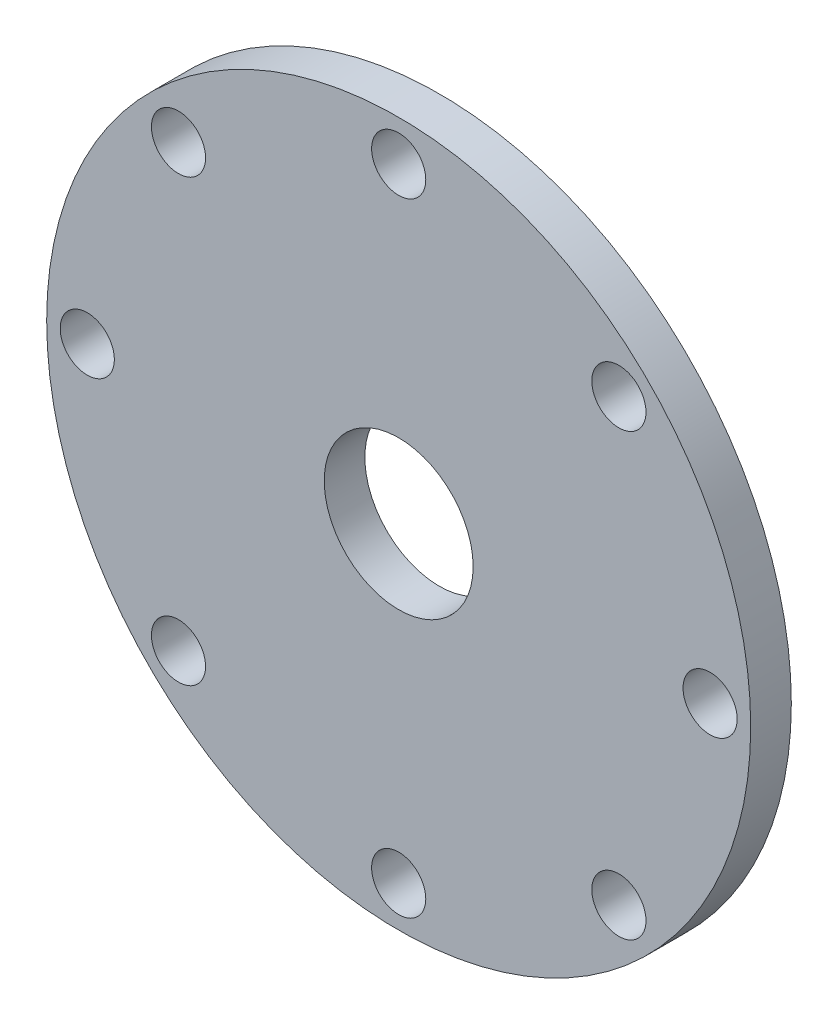
from build123d import *

# Parameters (mm, degrees)
SKETCH2_R           = 130
SKETCH2_R_2         = 27.5
BOSS_EXTRUDE1_DEPTH = 15
SKETCH3_R           = 10
CUT_EXTRUDE1_DEPTH  = 185.458667457
CIRPATTERN1_COUNT   = 8


with BuildPart() as part:
    # Sketch2 → Boss-Extrude1 (new body)
    with BuildSketch(Plane.XY):
        Circle(SKETCH2_R)
        Circle(SKETCH2_R_2, mode=Mode.SUBTRACT)
    extrude(amount=BOSS_EXTRUDE1_DEPTH)

    # Sketch3 → Cut-Extrude1 (cut, symmetric)
    with BuildSketch(Plane.XY):
        with Locations((-115, 0)):
            Circle(SKETCH3_R)
    cut_extrude1 = extrude(amount=CUT_EXTRUDE1_DEPTH, both=True, mode=Mode.SUBTRACT)

    # CirPattern1: Cut-Extrude1 ×8 about axis
    cirpattern1_axis = Axis((0, 0, 0), (0, 0, 1))
    for i in range(1, CIRPATTERN1_COUNT):
        add(cut_extrude1.rotate(cirpattern1_axis, i * 360 / CIRPATTERN1_COUNT), mode=Mode.SUBTRACT)


solid = part.part
